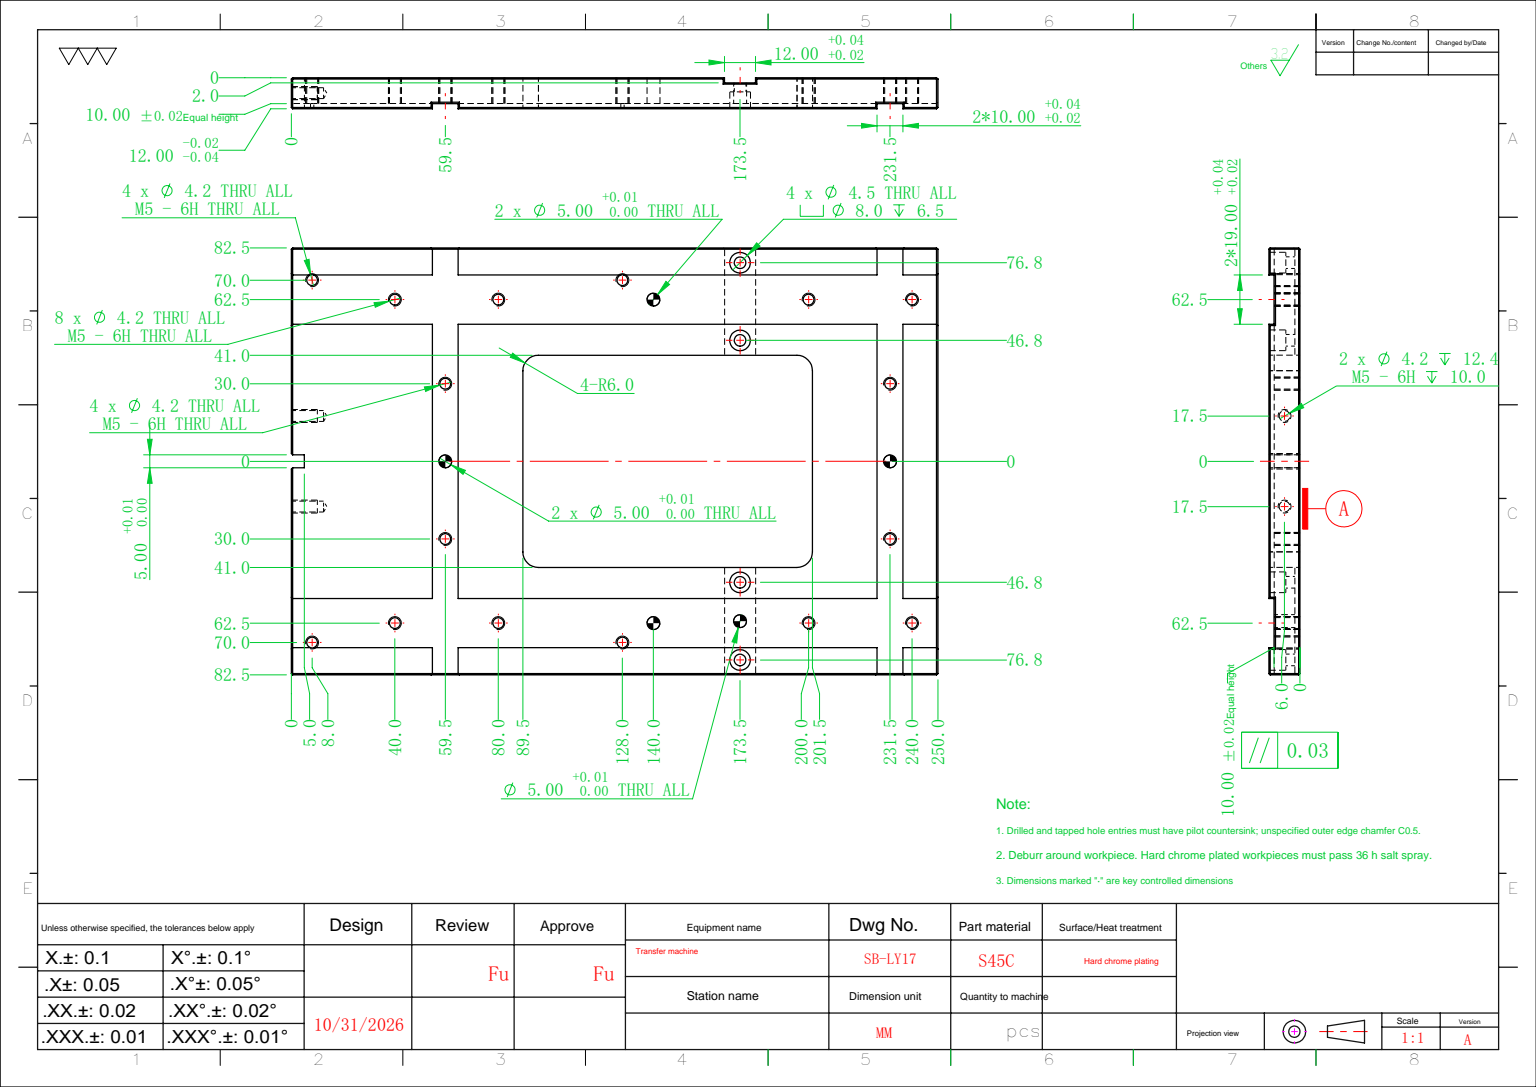
SolidWorks part; units mm, degrees
ref_plane "前视基准面" through (0, 0, 0) normal (0, 0, 1) x (1, 0, 0)
ref_plane "上视基准面" through (0, 0, 0) normal (0, 1, 0) x (1, 0, 0)
ref_plane "右视基准面" through (0, 0, 0) normal (1, 0, 0) x (0, 0, -1)
sketch "草图1" plane through (0, 0, 0) normal (0, 0, 1) x (1, 0, 0)
  line L1 (-82.5, -125) -> (82.5, -125)
  line L2 (-82.5, -125) -> (-82.5, 125)
  line L3 (-82.5, 125) -> (82.5, 125)
  line L4 (82.5, -125) -> (82.5, 125)
  line L5 (-82.5, -125) -> (82.5, 125) construction
  line L6 (-82.5, 125) -> (82.5, -125) construction
  point P0 (0, 0)
  dimension "D1" = 165
  dimension "D2" = 250
extrude "凸台-拉伸1" add sketch "草图1" along normal blind 12
sketch "草图2" plane through (0, 0, 0) normal (0, 0, -1) x (-1, 0, 0)
  line L0 (-82.5, 125) -> (82.5, 125) construction
  line L1 (72, 125) -> (53, 125)
  line L2 (72, 125) -> (72, -125)
  line L3 (72, -125) -> (53, -125)
  line L4 (53, 125) -> (53, -125)
  line L5 (0, 0) -> (0, 112.7425) construction
  line L6 (-53, 125) -> (-53, -125)
  line L7 (-72, -125) -> (-53, -125)
  line L8 (-72, 125) -> (-72, -125)
  line L9 (-72, 125) -> (-53, 125)
  line L10 (82.5, -125) -> (-82.5, -125) construction
  line L11 (62.5, 125) -> (62.5, 20.458) construction
  line L12 (-62.5, 125) -> (-62.5, 31.8535) construction
  dimension "D1" = 19
  dimension "D2" = 125
extrude "切除-拉伸1" cut sketch "草图2" against normal blind 2
sketch "草图3" plane through (0, 0, 0) normal (0, 0, -1) x (-1, 0, 0)
  line L0 (82.5, 125) -> (82.5, -125) construction
  line L1 (82.5, -70.5) -> (-82.5, -70.5)
  line L2 (82.5, -70.5) -> (82.5, -60.5)
  line L3 (82.5, -60.5) -> (-82.5, -60.5)
  line L4 (-82.5, -70.5) -> (-82.5, -60.5)
  line L5 (-82.5, -125) -> (-82.5, 125) construction
  line L7 (-82.5, -65.5) -> (116.0113, -65.5) construction
  line L8 (82.5, -125) -> (-82.5, -125) construction
  dimension "D1" = 10
  dimension "D2" = 59.5
extrude "切除-拉伸2" cut sketch "草图3" against normal blind 2
sketch "草图4" plane through (0, 0, 0) normal (0, 0, -1) x (-1, 0, 0)
  line L0 (82.5, 125) -> (82.5, -60.5) construction
  line L1 (82.5, 101.5) -> (-82.5, 101.5)
  line L2 (82.5, 101.5) -> (82.5, 111.5)
  line L3 (82.5, 111.5) -> (-82.5, 111.5)
  line L4 (-82.5, 101.5) -> (-82.5, 111.5)
  line L5 (-82.5, -60.5) -> (-82.5, 125) construction
  line L7 (-53, -70.5) -> (53, -70.5) construction
  dimension "D1" = 10
  dimension "D2" = 172
extrude "切除-拉伸3" cut sketch "草图4" against normal up to surface (2 mm away) up to face at (0, -39.3, 2)
hole_wizard "M5 螺纹孔1" positions "草图5" profile "草图6" tap size "M5" standard "ISO" end condition through all
sketch "草图5" plane through (0, 0, 0) normal (0, 0, -1) x (-1, 0, 0)
  line L0 (-82.5, 106.5) -> (82.5, 106.5) construction
  line L1 (-82.5, 111.5) -> (-82.5, 101.5) construction
  line L2 (82.5, 101.5) -> (82.5, 111.5) construction
  line L4 (82.5, -65.5) -> (-82.5, -65.5) construction
  line L5 (82.5, -70.5) -> (82.5, -60.5) construction
  line L6 (-82.5, -60.5) -> (-82.5, -70.5) construction
  line L8 (0, 106.5) -> (0, -65.5) construction
  point P0 (-29.9992, -65.5)
  point P3 (29.9992, -65.5)
  point P6 (29.9992, 106.5)
  point P9 (-29.9992, 106.5)
  dimension "D1" = 59.9985
sketch "草图6" plane through (29.9992, -65.5, 0) normal (1, 0, 0) x (0, 1, 0)
  line L0 (0, 0) -> (0, 12)
  line L1 (0, 12) -> (2.1, 12)
  line L2 (2.1, 12) -> (2.1, 0)
  line L5 (2.1, 0) -> (0, 0)
  line L11 (0, -6.35) -> (0, 107.95) construction
  dimension "通孔螺纹孔钻头直径" = 4.2
  dimension "通孔螺纹孔钻头深度" = 12
cosmetic thread "孔螺蚊线1" parameters "D2"=5
cosmetic thread "孔螺蚊线2" parameters "D2"=5
cosmetic thread "孔螺蚊线3" parameters "D2"=5
cosmetic thread "孔螺蚊线4" parameters "D2"=5
hole_wizard "大小mm 暗销孔1" positions "草图7" profile "草图8" hole size "Ø5.0" standard "ISO" end condition through all
sketch "草图7" plane through (0, 0, 2) normal (0, 0, -1) x (-1, 0, 0)
  line L0 (-29.9992, -65.5) -> (29.9992, -65.5) construction
  line L2 (-29.9992, 106.5) -> (29.9992, 106.5) construction
  point P0 (0, -65.5)
  point P16 (0, 106.5)
sketch "草图8" plane through (0, -65.5, 2) normal (1, 0, 0) x (0, 1, 0)
  line L0 (0, 0) -> (0, 10)
  line L1 (0, 10) -> (2.5, 10)
  line L2 (2.5, 10) -> (2.5, 0)
  line L5 (2.5, 0) -> (0, 0)
  line L11 (0, -6.35) -> (0, 107.95) construction
  dimension "通孔孔直径" = 5
  dimension "通孔孔深度" = 10
sketch "草图10" plane through (0, 0, 0) normal (0, 0, -1) x (-1, 0, 0)
  line L0 (35, -29.5) -> (35, 70.5) construction
  line L1 (29, -29.5) -> (29, 70.5)
  line L2 (41, -29.5) -> (41, 70.5)
  line L3 (82.5, -125) -> (-82.5, -125) construction
  line L4 (-35, -29.5) -> (-35, 70.5) construction
  line L5 (-29, -29.5) -> (-29, 70.5)
  line L6 (-41, -29.5) -> (-41, 70.5)
  line L7 (0, 41) -> (0, 0) construction
  line L8 (0, 20.5) -> (-123.048, 20.5) construction
  arc A0 (29, -29.5) -> (41, -29.5) centre (35, -29.5) ccw
  arc A1 (41, 70.5) -> (29, 70.5) centre (35, 70.5) ccw
  arc A2 (-29, -29.5) -> (-41, -29.5) centre (-35, -29.5) cw
  arc A3 (-41, 70.5) -> (-29, 70.5) centre (-35, 70.5) cw
  point P2 (35, 20.5)
  point P12 (-35, 20.5)
  dimension "D3" = 100
  dimension "D4" = 145.5
  dimension "D1" = 70
  dimension "D2" = 12
extrude "切除-拉伸4" cut sketch "草图10" against normal through all
sketch "草图11" plane through (0, 0, 0) normal (0, 0, -1) x (-1, 0, 0)
  line L1 (35, -35.5) -> (-35, -35.5)
  line L2 (35, -35.5) -> (35, 76.5)
  line L3 (35, 76.5) -> (-35, 76.5)
  line L4 (-35, -35.5) -> (-35, 76.5)
  arc A0 (29, -29.5) -> (41, -29.5) centre (35, -29.5) ccw construction
  arc A1 (-29, 70.5) -> (-41, 70.5) centre (-35, 70.5) ccw construction
extrude "切除-拉伸5" cut sketch "草图11" against normal through all
sketch "草图13" plane through (0, 0, 12) normal (0, 0, 1) x (1, 0, 0)
  line L0 (-82.5, 125) -> (-82.5, -125) construction
  line L1 (-82.5, 54.5) -> (82.5, 54.5)
  line L2 (-82.5, 54.5) -> (-82.5, 42.5)
  line L3 (-82.5, 42.5) -> (82.5, 42.5)
  line L4 (82.5, 54.5) -> (82.5, 42.5)
  line L5 (82.5, -125) -> (82.5, 125) construction
  line L6 (-82.5, -125) -> (82.5, -125) construction
  line L8 (-66, 48.5) -> (117.0995, 48.5) construction
  dimension "D1" = 12
  dimension "D2" = 173.5
extrude "切除-拉伸6" cut sketch "草图13" against normal blind 2
hole_wizard "M5 螺纹孔2" positions "草图14" profile "草图15" tap size "M5" standard "ISO" end condition through all
sketch "草图14" plane through (0, 0, 12) normal (0, 0, 1) x (1, 0, 0)
  line L8 (0, 0) -> (0, -153.5852) construction
  line L12 (82.5, 125) -> (-82.5, 125) construction
  point P0 (-70, 3)
  point P2 (-70, -117)
  point P29 (70, 3)
  point P32 (70, -117)
  dimension "D1" = 140
  dimension "D2" = 120
  dimension "D3" = 122
sketch "草图15" plane through (-70, 3, 12) normal (1, 0, 0) x (0, -1, 0)
  line L0 (0, 0) -> (0, 12)
  line L1 (0, 12) -> (2.1, 12)
  line L2 (2.1, 12) -> (2.1, 0)
  line L5 (2.1, 0) -> (0, 0)
  line L11 (0, -6.35) -> (0, 107.95) construction
  dimension "通孔螺纹孔钻头直径" = 4.2
  dimension "通孔螺纹孔钻头深度" = 12
cosmetic thread "孔螺蚊线6" parameters "D2"=5
cosmetic thread "孔螺蚊线8" parameters "D2"=5
cosmetic thread "孔螺蚊线20" parameters "D2"=5
cosmetic thread "孔螺蚊线21" parameters "D2"=5
hole_wizard "M4 六角凹头螺钉的柱形沉头孔1" positions "草图16" profile "草图17" counterbore size "M4" standard "ISO" end condition through all
sketch "草图16" plane through (0, 0, 0) normal (0, 0, -1) x (-1, 0, 0)
  line L3 (41, 48.5) -> (82.5, 48.5) construction
  line L4 (82.5, 54.5) -> (82.5, 42.5) construction
  line L5 (41, 42.5) -> (41, 54.5) construction
  line L6 (61.75, 54.5) -> (61.75, 33.9174) construction
  line L7 (41, 54.5) -> (82.5, 54.5) construction
  line L8 (0, 0) -> (0, 141.5399) construction
  point P0 (46.75, 48.5)
  point P2 (76.75, 48.5)
  point P39 (-76.75, 48.5)
  point P40 (-46.75, 48.5)
  dimension "D1" = 30
sketch "草图17" plane through (-46.75, 48.5, 0) normal (1, 0, 0) x (0, 1, 0)
  line L0 (0, 0) -> (0, 12)
  line L1 (0, 12) -> (2.25, 12)
  line L3 (2.25, 12) -> (2.25, 6.5)
  line L4 (2.25, 6.5) -> (4, 6.5)
  line L5 (4, 6.5) -> (4, 0)
  line L7 (4, 0) -> (0, 0)
  line L11 (0, -6.35) -> (0, 107.95) construction
  dimension "通孔孔直径" = 4.5
  dimension "通孔孔深度" = 12
  dimension "柱形沉头孔直径" = 8
  dimension "柱形沉头孔深度" = 6.5
hole_wizard "大小mm 暗销孔2" positions "草图18" profile "草图19" hole size "Ø5.0" standard "ISO" end condition through all
sketch "草图18" plane through (0, 0, 2) normal (0, 0, -1) x (-1, 0, 0)
  line L0 (46.75, 48.5) -> (76.75, 48.5) construction
  point P0 (61.75, 48.5)
sketch "草图19" plane through (-61.75, 48.5, 2) normal (1, 0, 0) x (0, 1, 0)
  line L0 (0, 0) -> (0, 10)
  line L1 (0, 10) -> (2.5, 10)
  line L2 (2.5, 10) -> (2.5, 0)
  line L5 (2.5, 0) -> (0, 0)
  line L11 (0, -6.35) -> (0, 107.95) construction
  dimension "通孔孔直径" = 5
  dimension "通孔孔深度" = 10
hole_wizard "M5 螺纹孔3" positions "草图20" profile "草图21" tap size "M5" standard "ISO"
sketch "草图20" plane through (0, -125, 0) normal (0, -1, 0) x (-1, 0, 0)
  line L0 (0, 0) -> (0, -12) construction
  line L1 (82.5, -12) -> (-82.5, -12) construction
  point P0 (-17.5, -6)
  point P3 (17.5, -6)
  dimension "D1" = 35
  dimension "D2" = 6
sketch "草图21" plane through (17.5, -125, 6) normal (1, 0, 0) x (0, 0, -1)
  line L0 (0, 0) -> (0, 13.6618)
  line L1 (0, 13.6618) -> (2.1, 12.4)
  line L2 (2.1, 12.4) -> (2.1, 0)
  line L5 (2.1, 0) -> (0, 0)
  line L10 (0, 13.6618) -> (-2.1, 12.4) construction
  line L11 (0, -6.35) -> (0, 107.95) construction
  dimension "螺纹孔钻头直径" = 4.2
  dimension "螺纹孔钻头深度" = 12.4
  dimension "导头角度" = 118
cosmetic thread "孔螺蚊线9" parameters "D1"=10, "D2"=5
cosmetic thread "孔螺蚊线10" parameters "D1"=10, "D2"=5
sketch "草图22" plane through (0, -125, 0) normal (0, -1, 0) x (1, 0, 0)
  line L0 (-82.5, 12) -> (82.5, 12) construction
  line L1 (-2.5, 12) -> (2.5, 12)
  line L2 (-2.5, 12) -> (-2.5, 0)
  line L3 (-2.5, 0) -> (2.5, 0)
  line L4 (2.5, 12) -> (2.5, 0)
  line L5 (-53, 0) -> (53, 0) construction
  line L6 (0, 0) -> (0, 15.7604) construction
  dimension "D1" = 5
extrude "切除-拉伸7" cut sketch "草图22" against normal blind 5
hole_wizard "M5 螺纹孔4" positions "草图23" profile "草图24" tap size "M5" standard "ISO" end condition through all
sketch "草图23" plane through (0, 0, 2) normal (0, 0, -1) x (-1, 0, 0)
  line L0 (62.5, 125) -> (62.5, -125) construction
  line L1 (72, 125) -> (53, 125) construction
  line L2 (53, -125) -> (72, -125) construction
  line L4 (-82.5, 125) -> (82.5, 125) construction
  line L5 (0, 0) -> (0, 53.9555) construction
  point P0 (62.5, -85)
  point P3 (62.5, -45)
  point P6 (62.5, 75)
  point P9 (62.5, 115)
  point P33 (-62.5, 115)
  point P34 (-62.5, 75)
  point P35 (-62.5, -45)
  point P36 (-62.5, -85)
  dimension "D1" = 10
  dimension "D2" = 40
  dimension "D3" = 120
  dimension "D4" = 40
sketch "草图24" plane through (-62.5, -85, 2) normal (1, 0, 0) x (0, 1, 0)
  line L0 (0, 0) -> (0, 10)
  line L1 (0, 10) -> (2.1, 10)
  line L2 (2.1, 10) -> (2.1, 0)
  line L5 (2.1, 0) -> (0, 0)
  line L11 (0, -6.35) -> (0, 107.95) construction
  dimension "通孔螺纹孔钻头直径" = 4.2
  dimension "通孔螺纹孔钻头深度" = 10
cosmetic thread "孔螺蚊线11" parameters "D2"=5
cosmetic thread "孔螺蚊线13" parameters "D2"=5
cosmetic thread "孔螺蚊线14" parameters "D2"=5
cosmetic thread "孔螺蚊线15" parameters "D2"=5
cosmetic thread "孔螺蚊线16" parameters "D2"=5
cosmetic thread "孔螺蚊线17" parameters "D2"=5
cosmetic thread "孔螺蚊线18" parameters "D2"=5
cosmetic thread "孔螺蚊线19" parameters "D2"=5
hole_wizard "大小mm 暗销孔3" positions "草图25" profile "草图26" hole size "Ø5.0" standard "ISO" end condition through all
sketch "草图25" plane through (0, 0, 2) normal (0, 0, -1) x (-1, 0, 0)
  line L0 (62.5, -45) -> (62.5, 75) construction
  line L2 (-62.5, -45) -> (-62.5, 75) construction
  point P0 (62.5, 15)
  point P15 (-62.5, 15)
sketch "草图26" plane through (-62.5, 15, 2) normal (1, 0, 0) x (0, 1, 0)
  line L0 (0, 0) -> (0, 10)
  line L1 (0, 10) -> (2.5, 10)
  line L2 (2.5, 10) -> (2.5, 0)
  line L5 (2.5, 0) -> (0, 0)
  line L11 (0, -6.35) -> (0, 107.95) construction
  dimension "通孔孔直径" = 5
  dimension "通孔孔深度" = 10
chamfer "倒角1" distance 0.5 angle 45 56 edges at (77.25, -125, 0) (72, -125, 1) (62.5, -125, 2) (53, -125, 1) (27.75, -125, 0) (2.5, -125, 6) (42.5, -125, 12) (-53, -125, 1) (-62.5, -125, 2) (-72, -125, 1) (-77.25, -125, 0) (-27.75, -125, 0) (-2.5, -125, 6) (-42.5, -125, 12) (-82.5, 42.5, 11) (-82.5, -41.25, 12) (-82.5, -125, 6) (-82.5, -97.75, 0) (-82.5, -70.5, 1) (-82.5, -65.5, 2) (-82.5, -60.5, 1) (-82.5, 20.5, 0) (-82.5, 101.5, 1) (-82.5, 106.5, 2) (-82.5, 111.5, 1) (-82.5, 118.25, 0) (-82.5, 48.5, 10) (-82.5, 54.5, 11) (-82.5, 89.75, 12) (-53, 125, 1) (0, 125, 0) (53, 125, 1) (62.5, 125, 2) (72, 125, 1) (77.25, 125, 0) (-62.5, 125, 2) (-72, 125, 1) (-77.25, 125, 0) (-82.5, 125, 6) (0, 125, 12) (82.5, 125, 6) (82.5, 118.25, 0) (82.5, 111.5, 1) (82.5, 106.5, 2) (82.5, 101.5, 1) (82.5, 20.5, 0) (82.5, -60.5, 1) (82.5, -65.5, 2) (82.5, -70.5, 1) (82.5, -97.75, 0) (82.5, -125, 6) (82.5, -41.25, 12) (82.5, 42.5, 11) (82.5, 48.5, 10) (82.5, 54.5, 11) (82.5, 89.75, 12)
